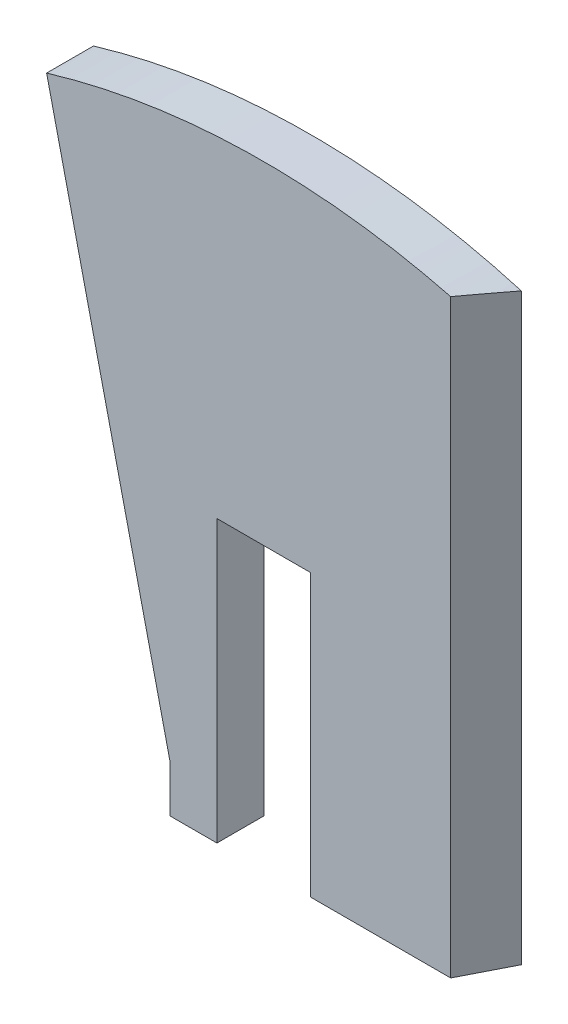
from build123d import *

# Parameters (mm, degrees)
BOSS_EXTRUDE1_DEPTH = 5
SKETCH2_W           = 20
SKETCH2_H           = 120
CUT_EXTRUDE1_DEPTH  = 10
CUT_EXTRUDE2_DEPTH  = 140.051478249


with BuildPart() as part:
    # Sketch1 → Boss-Extrude1 (new, symmetric)
    with BuildSketch(Plane.XY):
        with BuildLine():
            Line((-46.360690281, 154.180693982), (-20, 40))
            Line((-20, 40), (-20, 30))
            Line((-20, 30), (0, 30))
            Line((0, 30), (45, 30))
            Line((45, 30), (45, 40))
            Line((45, 40), (45, 154.583310872))
            ThreePointArc((45, 154.583310872), (-0.709503066, 160.998436655), (-46.360690281, 154.180693982))
        make_face()
    extrude(amount=BOSS_EXTRUDE1_DEPTH, both=True)

    # Sketch2 → Cut-Extrude1 (cut)
    with BuildSketch(Plane.XY.offset(5)):
        with Locations((0, 30)):
            Rectangle(SKETCH2_W, SKETCH2_H)
    extrude(amount=-CUT_EXTRUDE1_DEPTH, mode=Mode.SUBTRACT)

    # Sketch3 → Cut-Extrude2 (cut, through all)
    with BuildSketch(Plane.XZ.offset(-30)):
        Polygon((45, -5), (39.904745505, 5), (45, 5), align=None)
    extrude(amount=-CUT_EXTRUDE2_DEPTH, mode=Mode.SUBTRACT)


solid = part.part
